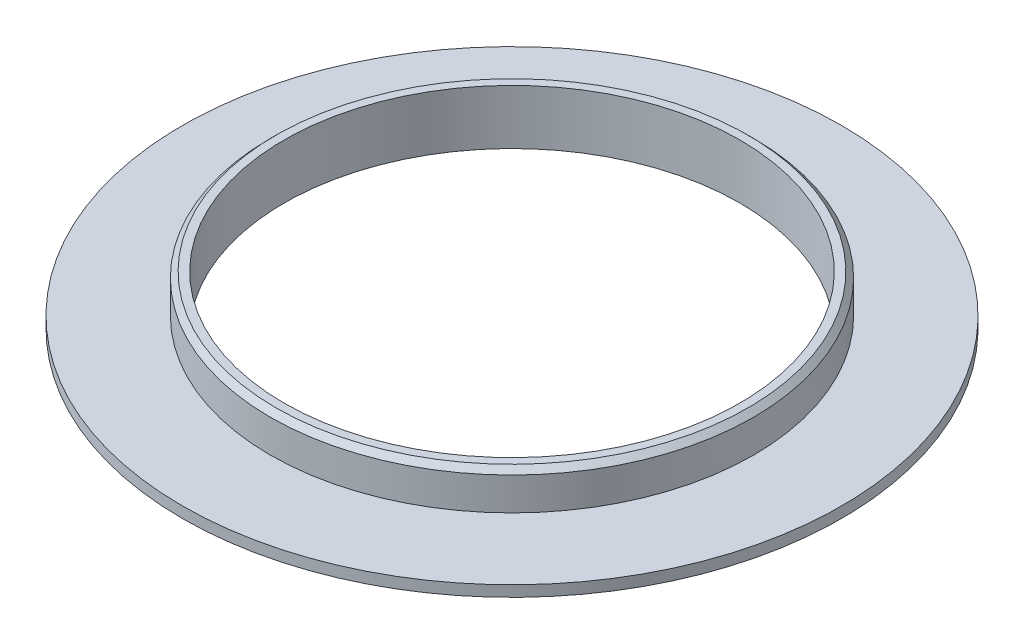
SolidWorks part; units mm, degrees
material "6061 合金"
ref_plane "前视基准面" through (0, 0, 0) normal (0, 0, 1) x (1, 0, 0)
ref_plane "上视基准面" through (0, 0, 0) normal (0, 1, 0) x (1, 0, 0)
ref_plane "右视基准面" through (0, 0, 0) normal (1, 0, 0) x (0, 0, -1)
sketch "草图1" plane through (0, 0, 0) normal (0, 1, 0) x (1, 0, 0)
  circle A0 centre (0, 0) radius 20.85
  circle A1 centre (0, 0) radius 30.1479
  dimension "D1" = 41.7
  dimension "D2" = 60.2958
extrude "凸台-拉伸1" add sketch "草图1" along normal blind 1.5
sketch "草图2" plane through (0, 1.5, 0) normal (0, 1, 0) x (1, 0, 0)
  circle A0 centre (0, 0) radius 20.85 construction
  circle A1 centre (0, 0) radius 20.85
  circle A2 centre (0, 0) radius 22.1
  dimension "D1" = 44.2
extrude "凸台-拉伸2" add sketch "草图2" along normal blind 3.5
chamfer "C0.5 倒角1" distance 0.5 angle 45 1 edges at (0, 5, 22.1)
chamfer "倒角2" distance 0.5 angle 75 1 edges at (0, 0, 30.1479)
